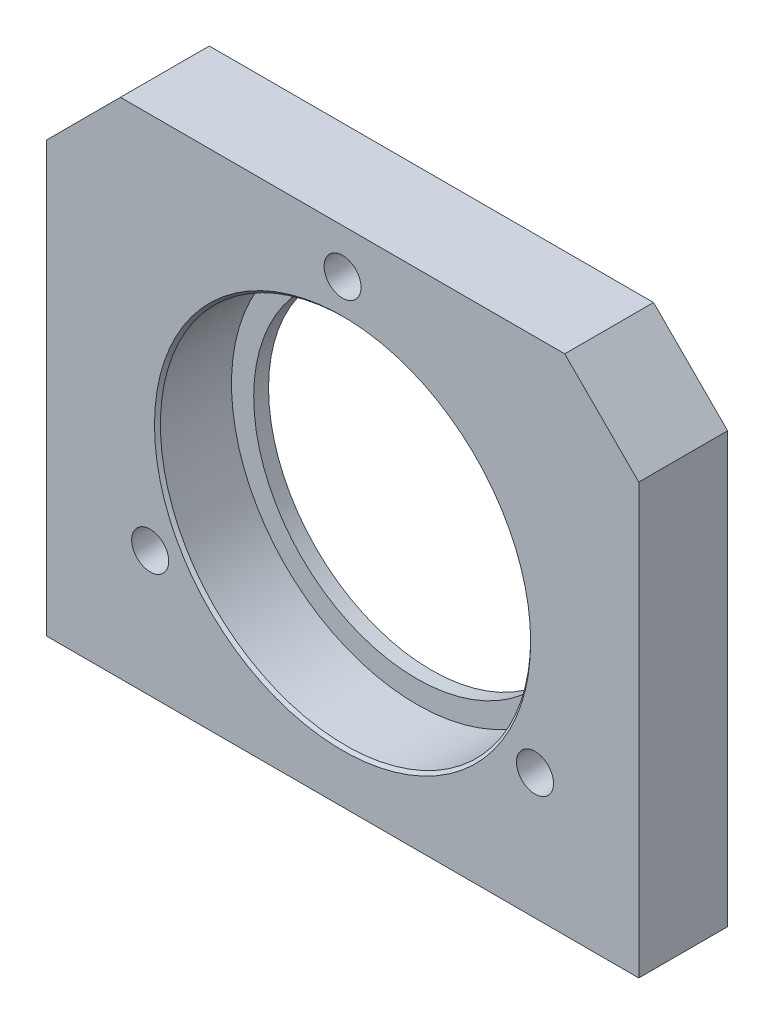
from build123d import *

# Parameters (mm, degrees)
SKETCH_1_R             = 11
EXTRUDE_1_DEPTH        = 6
SKETCH_2_R             = 12.5
CUT_EXTRUDE_1_DEPTH    = 5
HOLE_WIZARD_M3_1_D     = 2.5
HOLE_WIZARD_M3_2_D     = 2.5
HOLE_WIZARD_M3_2_DEPTH = 6
HOLE_WIZARD_M3_2_TIP   = 0.751075774
CHAMFER_1_SIZE         = 0.2


with BuildPart() as part:
    # 草图1 → 凸台-拉伸1 (new body)
    with BuildSketch(Plane.XY):
        Polygon((-20, -16), (20, -16), (20, 13), (15, 18), (-15, 18), (-20, 13), align=None)
        Circle(SKETCH_1_R, mode=Mode.SUBTRACT)
    extrude(amount=EXTRUDE_1_DEPTH)

    # 草图2 → 切除-拉伸1 (cut)
    with BuildSketch(Plane.XY.offset(6)):
        Circle(SKETCH_2_R)
    extrude(amount=-CUT_EXTRUDE_1_DEPTH, mode=Mode.SUBTRACT)

    # M3 螺纹孔1 (through all)
    with Locations(Plane(origin=(0, 15.005632156, 6), x_dir=(1, 0, 0), z_dir=(0, 0, 1))):
        with Locations((0, 0), (-12.990381057, -22.505632156), (12.990381057, -22.505632156)):
            Hole(HOLE_WIZARD_M3_1_D / 2)

    # M3 螺纹孔2
    with Locations(Plane(origin=(-16, -16, 3), x_dir=(0, 0, -1), z_dir=(0, -1, 0))):
        with Locations((0, 0), (0, 32)):
            Hole(HOLE_WIZARD_M3_2_D / 2, depth=HOLE_WIZARD_M3_2_DEPTH)
            with Locations((0, 0, -(HOLE_WIZARD_M3_2_DEPTH + HOLE_WIZARD_M3_2_TIP / 2))):  # 118° drill point
                Cone(0, HOLE_WIZARD_M3_2_D / 2, HOLE_WIZARD_M3_2_TIP, mode=Mode.SUBTRACT)

    # 倒角1
    chamfer_1_edges = [part.edges().sort_by_distance(p)[0] for p in [
        (-12.5, 0, 6),
    ]]
    chamfer(chamfer_1_edges, length=CHAMFER_1_SIZE)


solid = part.part
